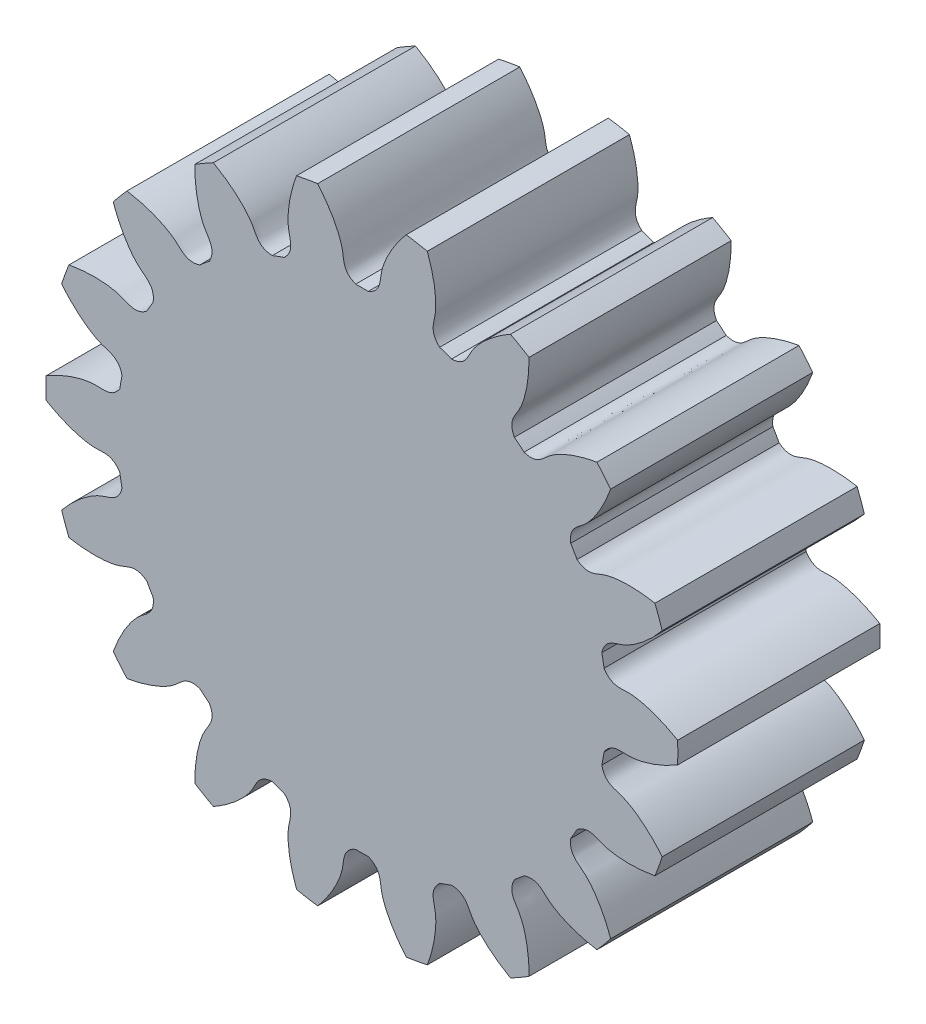
from build123d import *

# Parameters (mm, degrees)
SKETCH1_R           = 12.5
BOSS_EXTRUDE1_DEPTH = 8
CUT_EXTRUDE1_DEPTH  = 20.403607912
CIRPATTERN1_COUNT   = 18


with BuildPart() as part:
    # Sketch1 → Boss-Extrude1 (new body)
    with BuildSketch(Plane.XY):
        Circle(SKETCH1_R)
    extrude(amount=BOSS_EXTRUDE1_DEPTH)

    # Sketch2 → Cut-Extrude1 (cut, through all)
    with BuildSketch(Plane.XY):
        with BuildLine():
            ThreePointArc((0.249254449, 9.684292874), (0, 9.6875), (-0.249254449, 9.684292874))
            add(Edge.make_bspline(
                [(-0.249254449, 9.684292874), (-0.76888005, 9.898350488), (-0.703486312, 10.298374378), (-0.789791143, 10.678244321), (-0.7984394, 10.713133251), (-0.808884492, 10.751925593), (-0.821280887, 10.794562728), (-0.835787538, 10.84098021), (-0.852559647, 10.891109165), (-0.871751067, 10.944875915), (-0.893513396, 11.002202161), (-0.917996094, 11.063004996), (-0.945346283, 11.127196973), (-0.975708651, 11.194686165), (-1.009225323, 11.265376225), (-1.046035746, 11.339166457), (-1.086276569, 11.41595188), (-1.130081531, 11.495623304), (-1.177581345, 11.578067405), (-1.228903588, 11.663166799), (-1.28417259, 11.750800128), (-1.343509328, 11.84084214), (-1.407031319, 11.933163775), (-1.474852518, 12.027632257), (-1.547083214, 12.124111182), (-1.623829934, 12.222460613), (-1.705195343, 12.32253718), (-1.791278154, 12.424194171), (-1.882173032, 12.527281643), (-1.977970504, 12.631646517), (-2.078756878, 12.737132691), (-2.184614151, 12.843581143), (-2.295619932, 12.950830044), (-2.411847363, 13.05871487), (-2.533365041, 13.167068516), (-2.660236943, 13.275721413), (-2.792522359, 13.384501647), (-2.930275825, 13.493235075), (-3.073547051, 13.601745454), (-3.222380872, 13.709854557), (-3.376817155, 13.817382307), (-3.592594191, 13.961299395), (-3.759444298, 14.065417224), (-3.873201114, 14.133347975)],
                knots=[0, 0, 0, 0, 0.187591972, 0.192996016, 0.1991206, 0.205965723, 0.213531386, 0.221817587, 0.230824328, 0.240551609, 0.250999428, 0.262167787, 0.274056685, 0.286666122, 0.299996099, 0.314046614, 0.32881767, 0.344309264, 0.360521397, 0.37745407, 0.395107283, 0.413481034, 0.432575325, 0.452390155, 0.472925524, 0.494181432, 0.51615788, 0.538854867, 0.562272393, 0.586410459, 0.611269064, 0.636848208, 0.663147891, 0.690168114, 0.717908876, 0.746370177, 0.775552017, 0.805454397, 0.836077316, 0.867420774, 0.899484772, 0.932269309, 1, 1, 1, 1], degree=3))
            ThreePointArc((-3.873201114, 14.133347975), (0, 14.654460476), (3.873201114, 14.133347975))
            add(Edge.make_bspline(
                [(0.249254449, 9.684292874), (0.76888005, 9.898350488), (0.703486312, 10.298374378), (0.789791143, 10.678244321), (0.7984394, 10.713133251), (0.808884492, 10.751925593), (0.821280887, 10.794562728), (0.835787538, 10.84098021), (0.852559647, 10.891109165), (0.871751067, 10.944875915), (0.893513396, 11.002202161), (0.917996094, 11.063004996), (0.945346283, 11.127196973), (0.975708651, 11.194686165), (1.009225323, 11.265376225), (1.046035746, 11.339166457), (1.086276569, 11.41595188), (1.130081531, 11.495623304), (1.177581345, 11.578067405), (1.228903588, 11.663166799), (1.28417259, 11.750800128), (1.343509328, 11.84084214), (1.407031319, 11.933163775), (1.474852518, 12.027632257), (1.547083214, 12.124111182), (1.623829934, 12.222460613), (1.705195343, 12.32253718), (1.791278154, 12.424194171), (1.882173032, 12.527281643), (1.977970504, 12.631646517), (2.078756878, 12.737132691), (2.184614151, 12.843581143), (2.295619932, 12.950830044), (2.411847363, 13.05871487), (2.533365041, 13.167068516), (2.660236943, 13.275721413), (2.792522359, 13.384501647), (2.930275825, 13.493235075), (3.073547051, 13.601745454), (3.222380872, 13.709854557), (3.376817155, 13.817382307), (3.592594191, 13.961299395), (3.759444298, 14.065417224), (3.873201114, 14.133347975)],
                knots=[0, 0, 0, 0, 0.187591972, 0.192996016, 0.1991206, 0.205965723, 0.213531386, 0.221817587, 0.230824328, 0.240551609, 0.250999428, 0.262167787, 0.274056685, 0.286666122, 0.299996099, 0.314046614, 0.32881767, 0.344309264, 0.360521397, 0.37745407, 0.395107283, 0.413481034, 0.432575325, 0.452390155, 0.472925524, 0.494181432, 0.51615788, 0.538854867, 0.562272393, 0.586410459, 0.611269064, 0.636848208, 0.663147891, 0.690168114, 0.717908876, 0.746370177, 0.775552017, 0.805454397, 0.836077316, 0.867420774, 0.899484772, 0.932269309, 1, 1, 1, 1], degree=3))
        make_face()
    cut_extrude1 = extrude(amount=CUT_EXTRUDE1_DEPTH, mode=Mode.SUBTRACT)

    # CirPattern1: Cut-Extrude1 ×18 about axis
    cirpattern1_axis = Axis((0, 0, -0.4), (0, 0, 1))
    for i in range(1, CIRPATTERN1_COUNT):
        add(cut_extrude1.rotate(cirpattern1_axis, i * 360 / CIRPATTERN1_COUNT), mode=Mode.SUBTRACT)


solid = part.part
